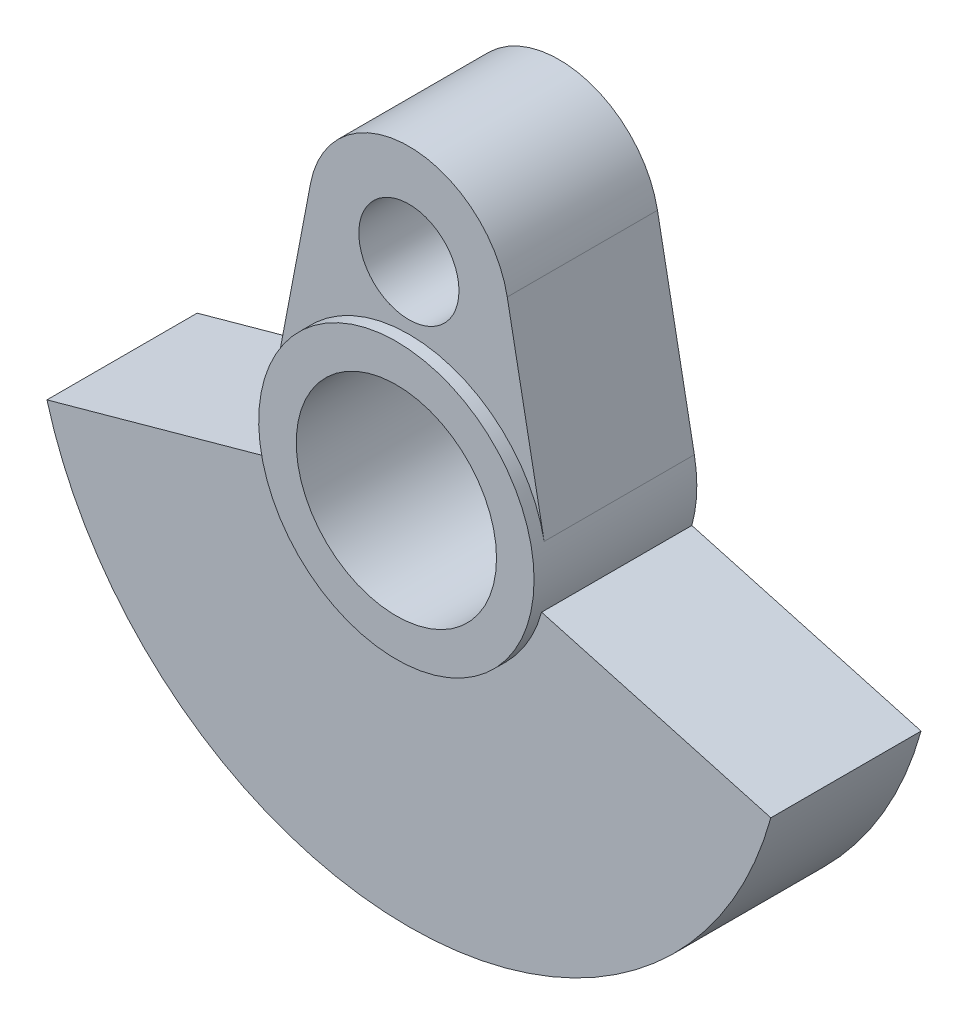
SolidWorks part; units mm, degrees
ref_plane "Front Plane" through (0, 0, 0) normal (0, 0, 1) x (1, 0, 0)
ref_plane "Top Plane" through (0, 0, 0) normal (0, 1, 0) x (1, 0, 0)
ref_plane "Right Plane" through (0, 0, 0) normal (1, 0, 0) x (0, 0, -1)
other "Configuration Table"
sketch "Sketch1" plane through (0, 0, 0) normal (0, 0, 1) x (1, 0, 0)
  line L0 (0, -4) -> (0, -15) construction
  line L1 (-5.3008, -1.4667) -> (-14.4568, -4)
  line L2 (5.3008, -1.4667) -> (14.4568, -4)
  arc A0 (-14.4568, -4) -> (14.4568, -4) centre (0, 0) ccw
  arc A2 (5.3008, -1.4667) -> (-5.3008, -1.4667) centre (0, 0) ccw
  circle A3 centre (0, 0) radius 4
  dimension "D1" = 30
  dimension "D3" = 11
  dimension "D4" = 8
  dimension "D2" = 4
extrude "Boss-Extrude2" add sketch "Sketch1" along normal blind 6 contours L2 A0 L1 A2
sketch "Sketch3" plane through (0, 0, 0) normal (0, 0, 1) x (1, 0, 0)
  line L0 (-3.9291, 8.75) -> (-5.4025, 1.0313)
  line L1 (0, 0) -> (0, 4) construction
  line L2 (3.9291, 8.75) -> (5.4025, 1.0313)
  line L3 (0, 5.5) -> (0, 8) construction
  circle A0 centre (0, 8) radius 2
  arc A1 (3.9291, 8.75) -> (-3.9291, 8.75) centre (0, 8) ccw
  arc A2 (5.3008, -1.4667) -> (-5.3008, -1.4667) centre (0, 0) ccw construction
  arc A3 (5.4025, 1.0313) -> (-5.4025, 1.0313) centre (0, 0) ccw
  dimension "D1" = 4
  dimension "D2" = 8
  dimension "D3" = 8
extrude "Boss-Extrude3" add sketch "Sketch3" along normal blind 6
sketch "Sketch4" plane through (0, 0, 6) normal (0, 0, 1) x (1, 0, 0)
  circle A0 centre (0, 0) radius 5.5
  circle A1 centre (0, 0) radius 4 construction
  circle A2 centre (0, 0) radius 4
  dimension "D1" = 11
extrude "Boss-Extrude4" add sketch "Sketch4" along normal blind 0.5 contours A0
